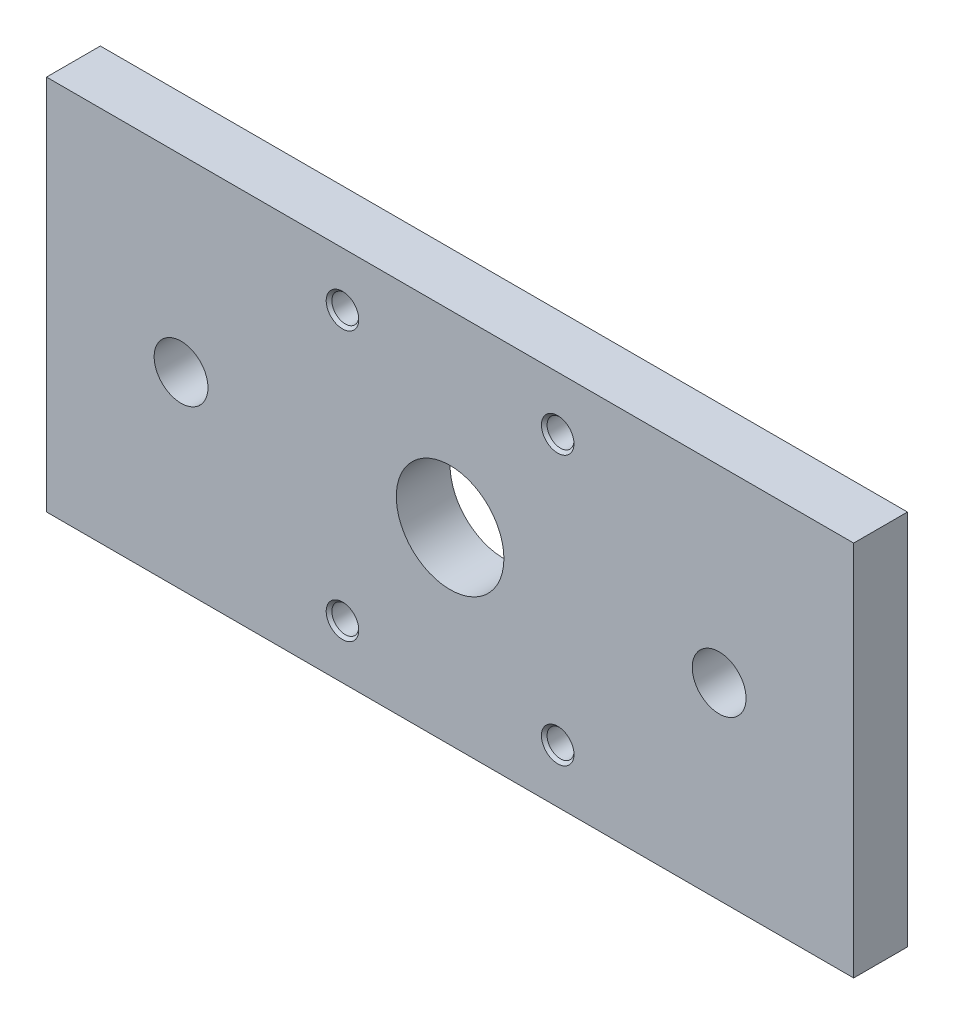
SolidWorks part; units mm, degrees
ref_plane "前视基准面" through (0, 0, 0) normal (0, 0, 1) x (1, 0, 0)
ref_plane "上视基准面" through (0, 0, 0) normal (0, 1, 0) x (1, 0, 0)
ref_plane "右视基准面" through (0, 0, 0) normal (1, 0, 0) x (0, 0, -1)
sketch "草图1" plane through (0, 0, 0) normal (0, 0, 1) x (1, 0, 0)
  line L1 (-75, 35) -> (75, 35)
  line L2 (-75, 35) -> (-75, -35)
  line L3 (-75, -35) -> (75, -35)
  line L4 (75, 35) -> (75, -35)
  line L5 (-75, 35) -> (75, -35) construction
  line L6 (-75, -35) -> (75, 35) construction
  point P0 (0, 0)
  dimension "D1" = 70
  dimension "D2" = 150
extrude "凸台-拉伸1" add sketch "草图1" along normal blind 10
sketch "草图2" plane through (0, 0, 10) normal (0, 0, 1) x (1, 0, 0)
  circle A0 centre (0, 0) radius 10
  dimension "D1" = 20
extrude "切除-拉伸1" cut sketch "草图2" against normal blind 55
sketch "草图7" plane through (0, 0, 10) normal (0, 0, 1) x (1, 0, 0)
  circle A0 centre (-50, 0) radius 5 construction
  circle A1 centre (50, 0) radius 5 construction
  circle A2 centre (-50, 0) radius 5
  circle A3 centre (50, 0) radius 5
extrude "切除-拉伸2" cut sketch "草图7" against normal blind 20
hole_wizard "M6 螺纹孔1" positions "草图8" profile "草图9" tap size "M6" standard "GB"
sketch "草图8" plane through (0, 0, 10) normal (0, 0, 1) x (1, 0, 0)
  point P0 (20, 25)
  point P3 (-20, 25)
  point P6 (-20, -25)
  point P9 (20, -25)
sketch "草图9" plane through (20, 25, 10) normal (1, 0, 0) x (0, -1, 0)
  line L0 (0, 0) -> (0, 15)
  line L1 (0, 15) -> (2.5, 13.4978)
  line L2 (2.5, 13.4978) -> (2.5, 0.525)
  line L3 (2.5, 0.525) -> (3.025, 0)
  line L5 (3.025, 0) -> (0, 0)
  line L6 (-2.5, 0.525) -> (-3.025, 0) construction
  line L10 (0, 15) -> (-2.5, 13.4978) construction
  line L11 (0, -6.35) -> (0, 107.95) construction
  dimension "螺纹孔钻头直径" = 5
  dimension "螺纹孔钻头深度" = 15
  dimension "近端锥形沉头孔直径" = 6.05
  dimension "近端锥形沉头孔角度" = 90
  dimension "导头角度" = 118
cosmetic thread "孔螺蚊线1" parameters "D1"=12, "D2"=6
cosmetic thread "孔螺蚊线2" parameters "D1"=12, "D2"=6
cosmetic thread "孔螺蚊线3" parameters "D1"=12, "D2"=6
cosmetic thread "孔螺蚊线4" parameters "D1"=12, "D2"=6
